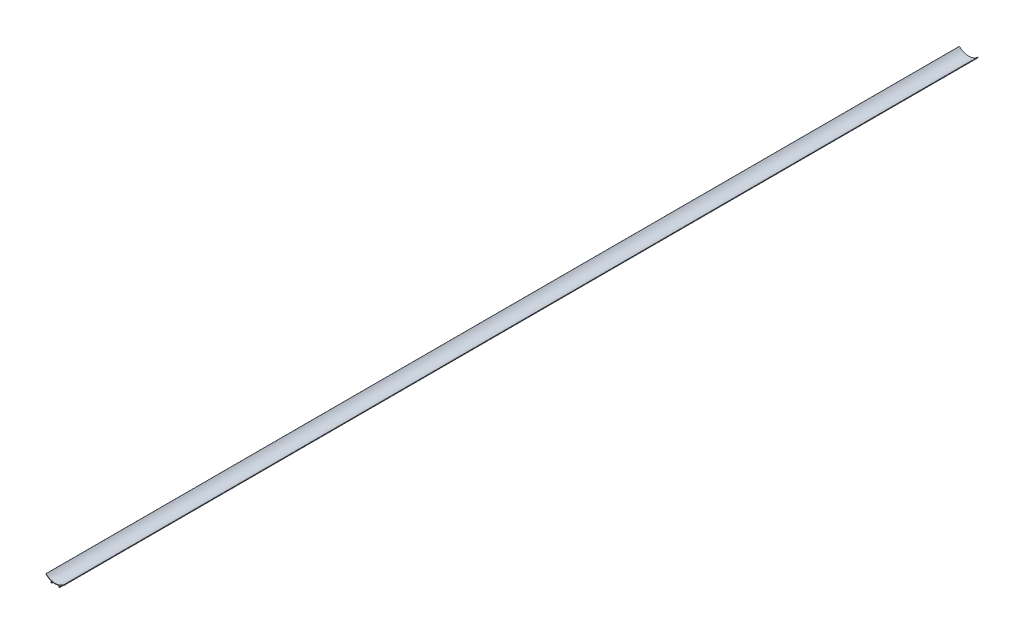
from build123d import *

# Parameters (mm, degrees)
EXTRUDE_1_DEPTH = 1145


with BuildPart() as part:
    # 草图2 → 凸台-拉伸1 (new, symmetric)
    with BuildSketch(Plane.XY):
        with BuildLine():
            Line((-11.25, 5.782842712), (-10.667157288, 5.199999999))
            Line((-10.667157288, 5.199999999), (-8.25, 5.199999999))
            Line((-8.25, 5.199999999), (-8.25, 6))
            Line((-8.25, 6), (-10.25, 6))
            Line((-10.25, 6), (-10.25, 7.726142057))
            Line((-10.25, 7.726142057), (-8.999999375, 7.724528349))
            Line((-8.999999375, 7.724528349), (-8.25, 8.473560125))
            Line((-8.25, 8.473560125), (-8.25, 8.88650173))
            ThreePointArc((-8.25, 8.88650173), (-5.642322013, 8.341793831), (-3, 8.002934636))
            Line((-3, 8.002934636), (-3, 7.70225919))
            Line((-3, 7.70225919), (3, 7.70225919))
            Line((3, 7.70225919), (3, 8.002934636))
            ThreePointArc((3, 8.002934636), (5.642322013, 8.341793831), (8.25, 8.88650173))
            Line((8.25, 8.88650173), (8.25, 8.473560125))
            Line((8.25, 8.473560125), (8.999999375, 7.724528349))
            Line((8.999999375, 7.724528349), (10.25, 7.726142057))
            Line((10.25, 7.726142057), (10.25, 6))
            Line((10.25, 6), (8.25, 6))
            Line((8.25, 6), (8.25, 5.2))
            Line((8.25, 5.2), (10.667157288, 5.2))
            Line((10.667157288, 5.2), (11.25, 5.782842712))
            Line((11.25, 5.782842712), (11.25, 9.785632758))
            ThreePointArc((11.25, 9.785632758), (17.712457567, 12.84892987), (23.391097866, 17.196364903))
            Line((23.391097866, 17.196364903), (23.391097866, 18.63499481))
            ThreePointArc((23.391097866, 18.63499481), (23.329308001, 18.727406852), (23.220298155, 18.705616343))
            ThreePointArc((23.220298155, 18.705616343), (0, 9.070311977), (-23.220298155, 18.705616342))
            ThreePointArc((-23.220298155, 18.705616342), (-23.329308002, 18.727406852), (-23.391097866, 18.634994809))
            Line((-23.391097866, 18.634994809), (-23.391097866, 17.196364902))
            ThreePointArc((-23.391097866, 17.196364902), (-17.712457568, 12.84892987), (-11.25, 9.785632758))
            Line((-11.25, 9.785632758), (-11.25, 5.782842712))
        make_face()
    extrude(amount=EXTRUDE_1_DEPTH, both=True)


solid = part.part
